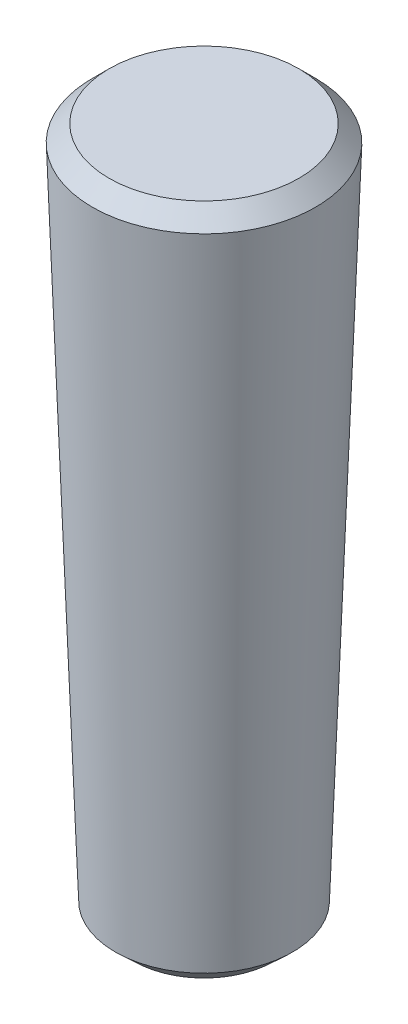
SolidWorks part; units mm, degrees
ref_plane "Front Plane" through (0, 0, 0) normal (0, 0, 1) x (1, 0, 0)
ref_plane "Top Plane" through (0, 0, 0) normal (0, 1, 0) x (1, 0, 0)
ref_plane "Right Plane" through (0, 0, 0) normal (1, 0, 0) x (0, 0, -1)
other "Configuration Table"
sketch "Sketch1" plane through (0, 0, 0) normal (0, 0, 1) x (1, 0, 0)
  line L0 (0, 0) -> (0, 54.622) construction
  line L1 (0, 0) -> (20.5706, 0) construction
  line L2 (0, 0) -> (0, 40)
  line L3 (0, 40) -> (6.5, 40)
  line L4 (0, 0) -> (5.1032, 0)
  line L5 (6.5, 40) -> (5.1426, 40)
  line L6 (6.5, 40) -> (5.1032, 0)
  line L7 (0, 40) -> (6.5, 40)
  line L8 (5.1032, 0) -> (0, 0)
revolve "Revolve4" add sketch "Sketch1" angle 360 about L0
chamfer "Chamfer1" distance 1 angle 45 2 edges at (0, 0, -5.1032) (0, 40, -6.5)
